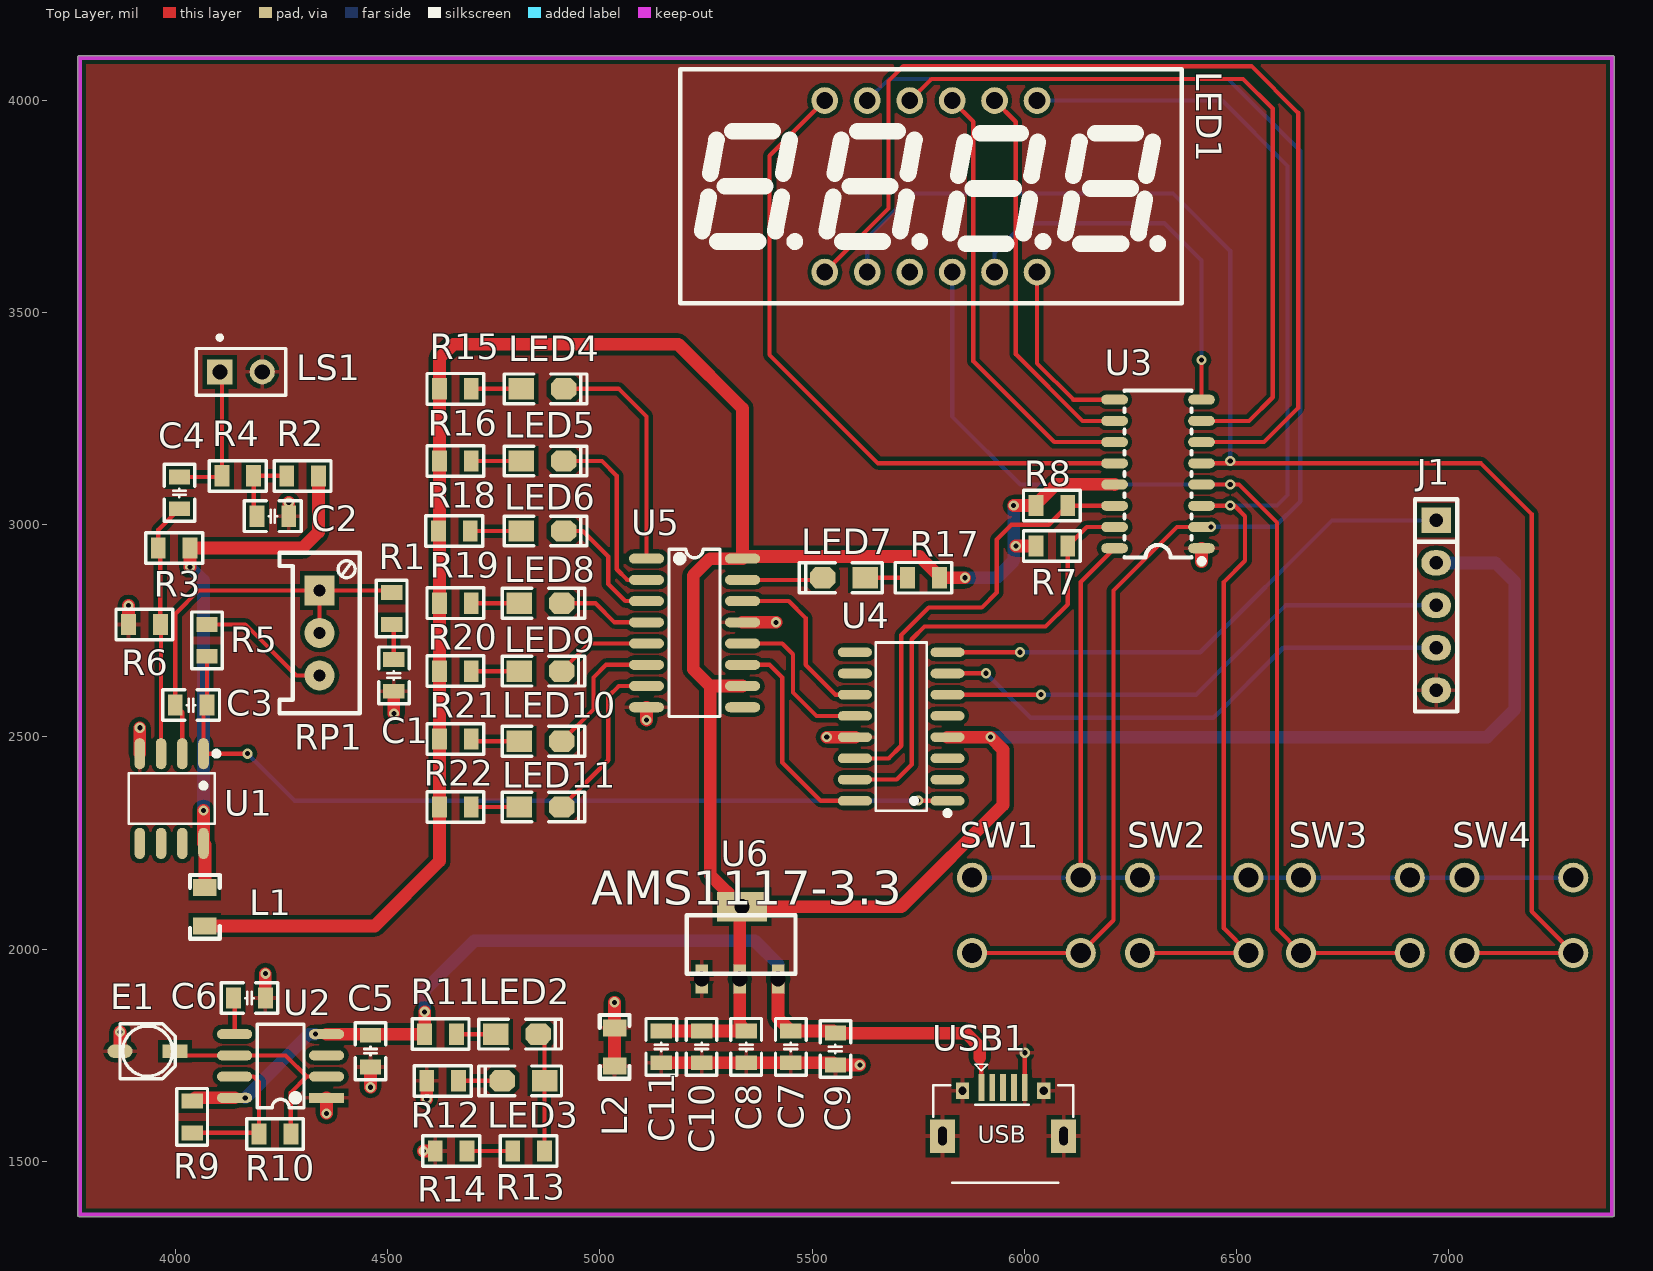
[diagram p0: Top Layer view]
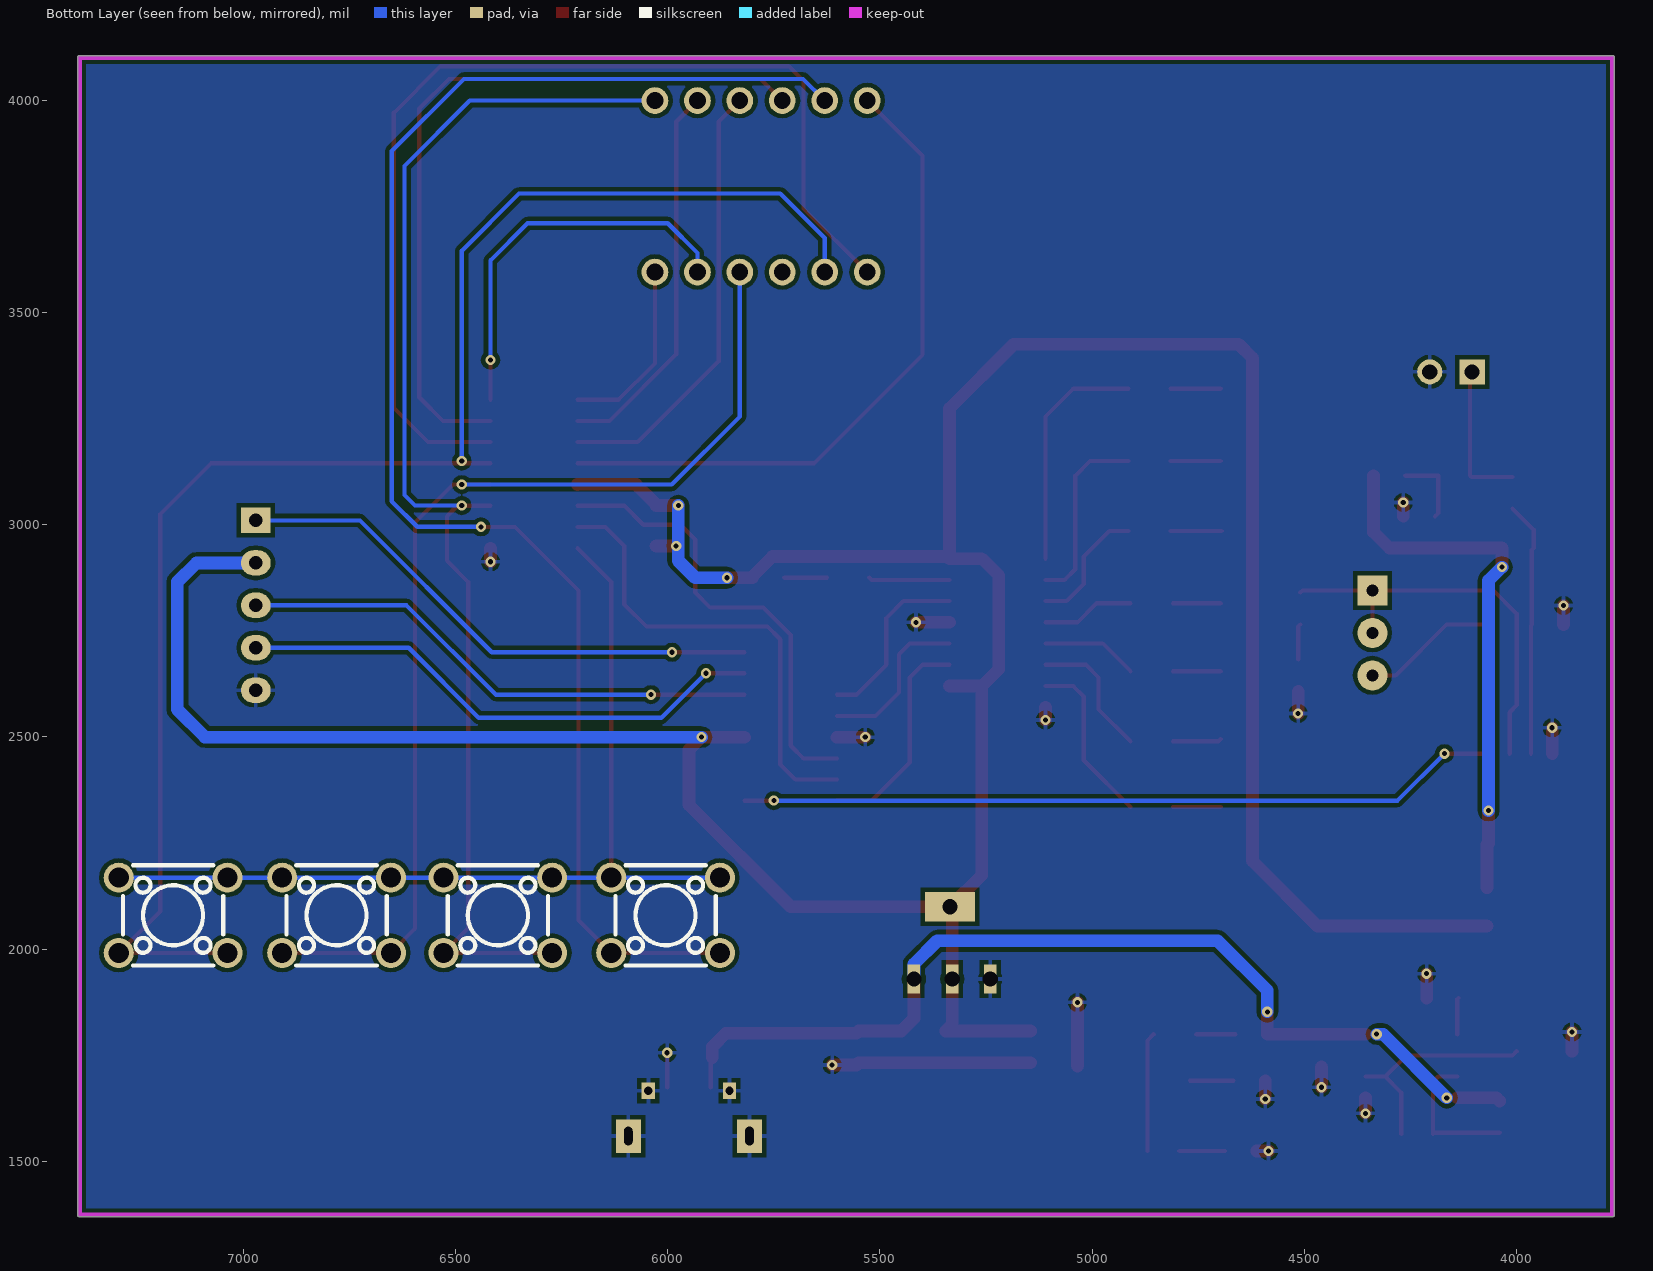
[diagram p1: Bottom Layer view, seen from below]
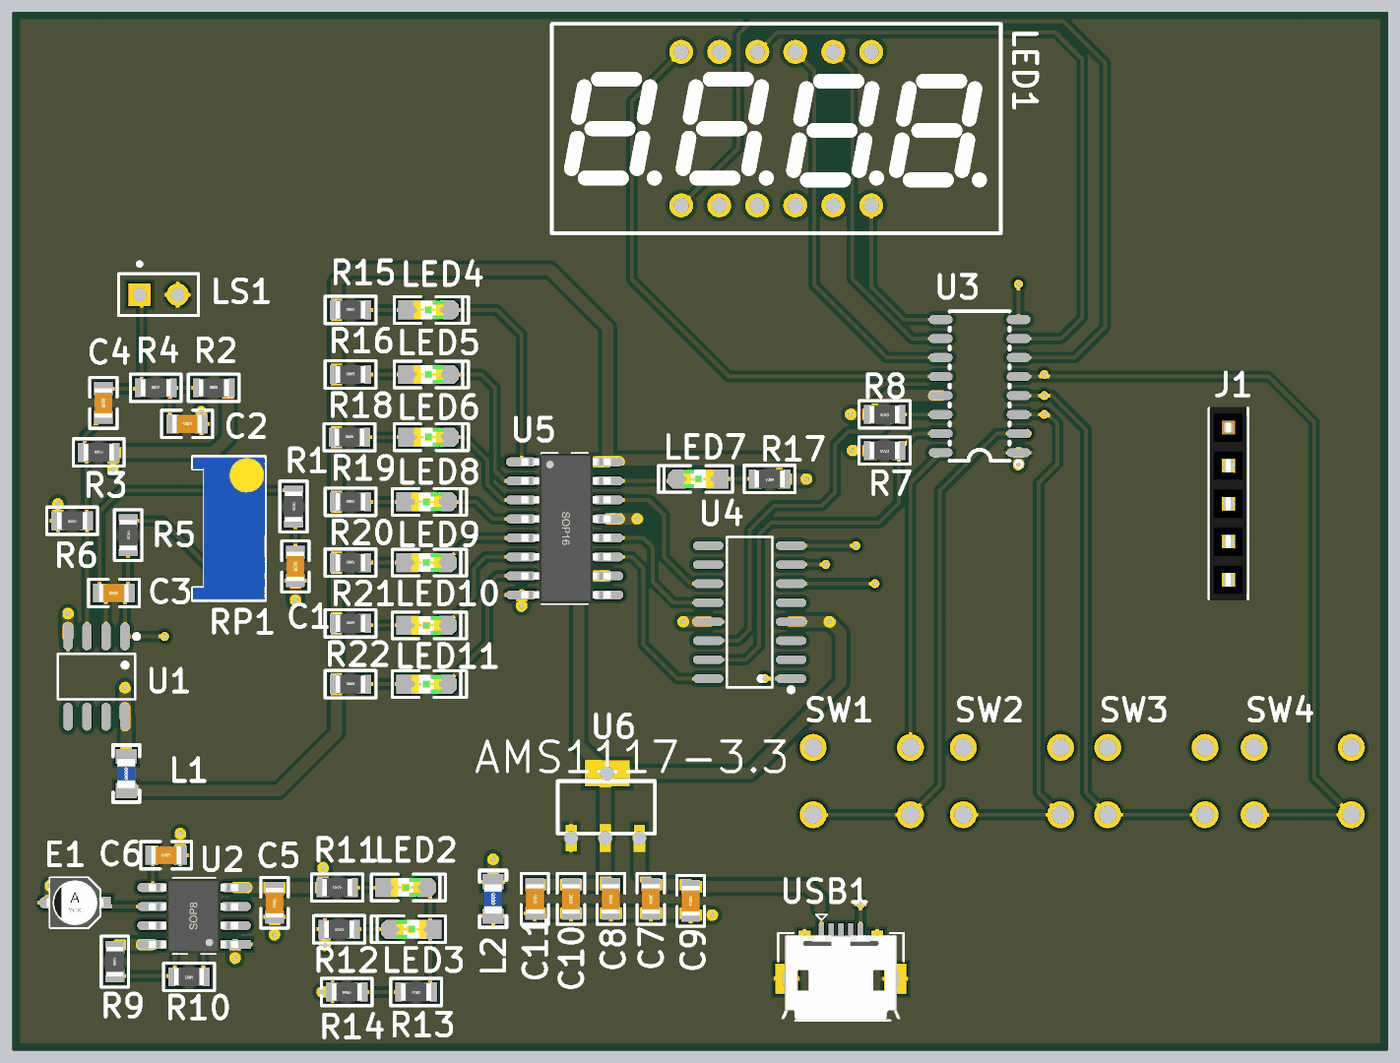
[diagram p2: 3D render of the assembled board from above, using the file's embedded part models]
# Altium PCB MISC80753.PcbDoc
Units mil, origin at the board's own origin, x right, y up, seen from the top; angles counter-clockwise.
Board outline 3620.03 x 2735.03 mil, 2 copper layers (Top Layer, Bottom Layer); 61 components, 56 nets, 207 pads, 36 vias.

## Layer stack, top to bottom (the 12.6 mil dielectric is the usual default, probably not edited)
Top Solder: solder mask 0.4, Solder Resist, Dk 3.5
Top Layer: signal copper 1.4
Dielectric 1: dielectric 12.6, FR-4, Dk 4.8
Bottom Layer: signal copper 1.4
Bottom Solder: solder mask 0.4, Solder Resist, Dk 3.5

## Board outline
3769.99,1375 ccw(c3775,1375) 3775,1369.98 7385,1369.98 ccw(c7385,1375) 7390.02,1375 7390.02,4100 ccw(c7385,4100) 7385,4105.02 3775,4105.02 ccw(c3775,4100) 3769.99,4100

## Design rules (kind name [scope] priority, off if disabled: settings)
Clearance [All] p1: gap=10
MinimumSolderMaskSliver [All] p1: minsoldermaskwidth=0
PolygonConnect [All] p1: connectstyle=Relief reliefconductorwidth=10 reliefentries=4 polygonreliefangle="90 Angle" airgapwidth=10
RoutingVias [All] p1: holewidth=28 width=50 viastyle="Through Hole" minholewidth=28 minwidth=50 maxholewidth=28 maxwidth=50
SilkToSilkClearance [All] p1: silktosilkclearance=0
SilkToSolderMaskClearance [IsPad] p1: minsilkscreentomaskgap=0 clearancetoexposedcopper=TRUE
SolderMaskExpansion [All] p1: expansion=4
Width [All] p1: maxlimit=30 minlimit=10 preferedwidth=10
27 further rules are at their usual default settings.

## Components (designator, comment, footprint, x,y, rotation, side; value= is the part's Value field where it differs from the comment)
C1 "10UF" "C 0805_L" 4515,2645 r270 top
C2 "0.1UF" "C 0805_L" 4230,3020 r180 top
C3 "100PF" "C 0805_L" 4037.4,2575 r0 top
C4 "0.01UF" "C 0805_L" 4010,3075 r270 top
C5 "10UF" "C 0805_L" 4460,1760 r90 top
C6 "10NF" "C 0805_L" 4175,1885 r0 top
C7 "100NF" "C 0805_L" 5450,1770 r90 top
C8 "100NF" "C 0805_L" 5345,1770 r90 top
C9 "10UF" "C 0805_L" 5555,1765 r90 top
C10 "10UF" "C 0805_L" 5240,1770 r90 top
C11 "100NF" "C 0805_L" 5145,1770 r90 top
E1 "10uF" "CM A(3*5.4)" 3935,1760 r0 top
J1 "Female HDR1X5" Fe-HDR1X5/2.54-S 6970,3010 r0 top
L1 "10uH" "L 0805" 4070,2100 r270 top
L2 "10uH" "L 0805" 5035,1770 r90 top
LED1 "SR410361N" LED-SEG-TH_12P-L30.0-W14.0-P2.54-S10.26-BL 5780,3796.97 r0 top
LED2 "Red" "LED 0805G" 4805,1800 r0 top
LED3 "Red" "LED 0805G" 4820,1690 r180 top
LED4 "Red" "LED 0805G" 4865,3320 r0 top
LED5 "Red" "LED 0805G" 4865,3150 r0 top
LED6 "Red" "LED 0805G" 4865,2985 r0 top
LED7 "Red" "LED 0805G" 5575,2875 r180 top
LED8 "Red" "LED 0805G" 4860,2815 r0 top
LED9 "Red" "LED 0805G" 4860,2655 r0 top
LED10 "Red" "LED 0805G" 4860,2490 r0 top
LED11 "Red" "LED 0805G" 4860,2335 r0 top
LS1 "Bell" PIN2 4105,3360 r0 top
R1 "1K" "R 0805_L" 4510,2802.6 r270 top
R2 "1K" "R 0805_L" 4300,3115 r0 top
R3 "1M" "R 0805_L" 3997.6,2945 r0 top
R4 "1K" "R 0805_L" 4147.4,3115 r0 top
R5 "10K" "R 0805_L" 4075,2727.4 r270 top
R6 "1M" "R 0805_L" 3927.6,2765 r180 top
R7 "10K" "R 0805_L" 6065,2950 r180 top
R8 "10K" "R 0805_L" 6065,3045 r180 top
R9 "100K" "R 0805_L" 4040,1605 r90 top
R10 "200K" "R 0805_L" 4235,1565 r180 top
R11 "1K" "R 0805_L" 4625,1800 r0 top
R12 "1K" "R 0805_L" 4630,1690 r180 top
R13 "10K" "R 0805_L" 4832.4,1525 r180 top
R14 "25K" "R 0805_L" 4650,1525 r180 top
R15 "1K" "R 0805_L" 4660,3320 r0 top
R16 "1K" "R 0805_L" 4660,3150 r0 top
R17 "1K" "R 0805_L" 5762.6,2875 r180 top
R18 "1K" "R 0805_L" 4657.4,2985 r0 top
R19 "1K" "R 0805_L" 4660,2815 r0 top
R20 "1K" "R 0805_L" 4660,2655 r0 top
R21 "1K" "R 0805_L" 4660,2495 r0 top
R22 "1K" "R 0805_L" 4660,2335 r0 top
RP1 "10K" 3296W 4340,2745 r270 top
SW1 "6x6x5" 四脚轻触开关 6005,2080 r0 top
SW2 "6x6x5" 四脚轻触开关 6400,2080 r0 top
SW3 "6x6x5" 四脚轻触开关 6780,2080 r0 top
SW4 "6x6x5" 四脚轻触开关 7165,2080 r0 top
U1 "COS2333SRC" SOP-8_L4.9-W3.9-P1.27-LS6.0-BL 3995,2355 r180 top
U2 "NE555" SOP8 4356.54,1650 r180 top
U3 "GN1651" SOP-16_L9.9-W3.9-P1.27-LS6.1-BL 6315,3115 r90 top
U4 "PY32F002AW15S6TU" SOP-16_L9.9-W3.9-P1.27-LS6.0-BL 5710,2520 r90 top
U5 "74HC595D" SOP16 5110,2920 r0 top
U6 "AMS1117-3.3" AMS1117-3.3 5222.95,2040.28 r0 top
USB1 "USB-5P" USB-MICRO_A 5950,1560 r0 top

## Footprints (in the part's own frame and the unit in brackets; to place one, negate y for a bottom-side part, rotate by r counter-clockwise, add the part's x,y. Pads: shape width x height; smd on the part's side, far side on the other; paste and mask are expansions set on the pad)
3296W [mm] "Precise Multi-Winding Adjustable Resistor"
  rect 1.8x1.8 hole 0.7: 1(-2.54,0)
  round 1.8 hole 0.7: 2(0,0) 3(2.54,0)
  silkscreen extent -4.8,-2.4 4.8,2.4, body extent -4.75,-2.4 4.75,2.4, height 11.52
AMS1117-3.3 [mm]
  rect 0.74x1.75 hole 0.914 paste+0 mask+0.051: 1(0.444,-2.801) 2(2.719,-2.801) 3(5.005,-2.801)
  rect 3x1.75 hole 0.914 paste+0 mask+0.051: 4(2.846,1.517)
  silkscreen extent -0.46,-2.49 6.04,1.01
"C 0805_L" [mil] "无极性贴片电容"
  rect 35x50 smd: 1(-37.4,0) 2(37.4,0)
  silkscreen extent -67,-36 67,36, body extent -39,-24 39,24, height 20
"CM A(3*5.4)" [mm] "贴片电解电容，直径3mm，高5.4mm"
  rect 1.5x0.8 smd: 1(1.651,0)
  oval 1.5x0.8 smd: 2(-1.65,0)
  silkscreen extent -1.65,-1.65 1.65,1.65, body extent -1.9,-1.65 1.9,1.65, height 5.4
Fe-HDR1X5/2.54-S [mil]
  rect 70x60 hole 32: 1(0,0)
  oval 70x60 hole 32: 2(0,-100) 3(0,-200) 4(0,-300) 5(0,-400)
  silkscreen extent -50,-450 50,50, body extent -50,-455 48,55, height 126
"L 0805" [mil] "小功率贴片电感"
  rect 40x55 smd: 1(-45,0) 2(45,0)
  silkscreen extent -75,-35 75,35, body extent -39,-24 39,24, height 35
"LED 0805G" [mil] "绿色0805LED"
  rect 60x50 smd: 1(-50,0)
  oct 60x50 smd: 2(50,0)
  silkscreen extent -90,-35 105,35, body extent -39,-25 39,25, height 32
LED-SEG-TH_12P-L30.0-W14.0-P2.54-S10.26-BL [mm]
  round 1.6 hole 1 paste+0 mask+0.051: 1(-6.35,-5.13) 2(-3.81,-5.13) 3(-1.27,-5.13) 4(1.27,-5.13) 5(3.81,-5.13) 6(6.35,-5.13) 7(6.35,5.13) 8(3.81,5.13) 9(1.27,5.13) 10(-1.27,5.13) 11(-3.81,5.13) 12(-6.35,5.13)
  silkscreen extent -15,-7 15,7
PIN2 [mm] "Photosensitive Diode; 2 Leads"
  rect 1.5x1.5 hole 0.9: 1(0,0)
  round 1.5 hole 0.9: 2(2.54,0)
  silkscreen extent -1.4,-1.4 3.94,2.17
"R 0805_L" [mil] "1/8W贴片电阻"
  rect 35x50 smd: 1(-37.4,0) 2(37.4,0)
  silkscreen extent -67,-36 67,36, body extent -39,-25 39,25, height 20
SOP8 [mm]
  rect 2.1x0.6 smd: 1(0,0)
  oval 2.1x0.6 smd: 2(0,-1.27) 3(0,-2.54) 4(0,-3.81) 5(5.5,-3.81) 6(5.5,-2.54) 7(5.5,-1.27) 8(5.5,0)
  silkscreen extent 1.35,-4.41 4.15,0.6, body extent -0.21,-4.4 5.8,0.6, height 1.9
SOP16 [mm]
  oval 2.1x0.6 smd: 1(0,0) 2(0,-1.27) 3(0,-2.54) 4(0,-3.81) 5(0,-5.08) 6(0,-6.35) 7(0,-7.62) 8(0,-8.89) 9(5.75,-8.89) 10(5.75,-7.62) 11(5.75,-6.35) 12(5.75,-5.08) 13(5.75,-3.81) 14(5.75,-2.54) 15(5.75,-1.27) 16(5.75,0)
  silkscreen extent 1.35,-9.45 4.4,0.56, body extent -0.04,-9.45 5.97,0.56, height 1.9
SOP-8_L4.9-W3.9-P1.27-LS6.0-BL [mm]
  oval 0.63x1.865 smd paste+0 mask+0.051: 1(-1.82,-2.682) 2(-0.55,-2.682) 3(0.72,-2.682) 4(1.99,-2.682) 5(1.99,2.682) 6(0.72,2.682) 7(-0.55,2.682) 8(-1.82,2.682)
  silkscreen extent -2.74,-2.83 2.66,1.52
SOP-16_L9.9-W3.9-P1.27-LS6.0-BL [mil]
  oval 22.6x80.24 smd paste+0 mask+2: 1(-170.43,-109.02) 2(-120.43,-109.02) 3(-70.43,-109.02) 4(-20.43,-109.02) 5(29.57,-109.02) 6(79.57,-109.02) 7(129.57,-109.02) 8(179.57,-109.02) 9(179.57,109.02) 10(129.57,109.02) 11(79.57,109.02) 12(29.57,109.02) 13(-20.43,109.02) 14(-70.43,109.02) 15(-120.43,109.02) 16(-170.43,109.02)
  silkscreen extent -205,-115 202,60
SOP-16_L9.9-W3.9-P1.27-LS6.1-BL [mm]
  oval 0.6x1.6 smd paste+0 mask+0.051: 1(-4.331,-2.6) 2(-3.061,-2.6) 3(-1.791,-2.6) 4(-0.521,-2.6) 5(0.749,-2.6) 6(2.019,-2.6) 7(3.289,-2.6) 8(4.559,-2.6) 9(4.559,2.6) 10(3.289,2.6) 11(2.019,2.6) 12(0.749,2.6) 13(-0.521,2.6) 14(-1.791,2.6) 15(-3.061,2.6) 16(-4.331,2.6)
  silkscreen extent -5.24,-2.76 5.11,2
USB-MICRO_A [mm] "micro型USB ，5.7*7.8*2.5mm"
  rect 0.35x1.6 smd: 1(-1.3,2.9) 2(-0.65,2.9) 3(0,2.9) 4(0.65,2.9) 5(1.3,2.9)
  rect 1.5x2 hole 0.5 slot 1.1 at 90 deg: 5(-3.625,0) 5(3.625,0)
  rect 0.8x1 hole 0.5: 5(-2.425,2.71) 5(2.425,2.71)
  silkscreen extent -4.19,-2.79 4.19,4.3, body extent -4,-2.71 4,2.89, height 2.8
四脚轻触开关 [mm]
  round 1.8 hole 1.2 paste+0 mask+0.102: 1(3.25,2.25) 2(-3.25,2.25) 3(3.25,-2.25) 4(-3.25,-2.25)

## Part data
C1 C2 C3 C4 C5 C6 C7 C8 C9 C10 C11: library part C, "Chip capacitor"
E1: library part CE_SMD, "Chip electrolytic capacitor"
L1 L2: library part L, "Low-power chip inductor"
LED2 LED3 LED4 LED5 LED6 LED7 LED8 LED9 LED10 LED11: library part LED-SMD, "Chip LED"
LS1: "Electrical Bell"
R1 R2 R3 R4 R5 R6 R7 R8 R9 R10 R11 R12 R13 R14 R15 R16 R17 R18 R19 R20 R21 R22: library part R, "Chip resistor"
RP1: library part RP, "Single-gang potentiometer"
SW1 SW2 SW3 SW4: library part "TSW DIP-6x6", "Through-hole 6x6 tactile switch"
U2: library part NE555D, "General-Purpose Single Bipolar Timer"
U5: library part SN74HC595D, "8-Bit Shift Register with 3-State Output Registers"
USB1: "Micro USB female socket"

## Via types
v1: diameter 24, hole 12, Top Layer to Bottom Layer, 36 vias

## Nets (pads, with @x,y where several pads share a name; then routed paths per layer and width w, separated by ;. In a path a pad name is that pad's centre, name@x,y a point inside that pad or via, vN(x,y) a via of type N, cw(c..) or ccw(c..) an arc to the next point about the centre after c; other vN are vias at no path point)
3V3: C8.2 C10.2 C11.2 J1.2 L1.2 R7.2 R8.2 R15.1 R16.1 R17.1 R18.1 R19.1 R20.1 R21.1 R22.1 U3.13 U4.4 U5.10 U5.16 U6.2 U6.4 | length 8351.1
  Top Layer w30: L1.2 4470,2055 4622.6,2207.6 R22.1 R21.1 R20.1 R19.1 R16.1 R15.1 4622.6,3392.6 4655,3425 5185,3425 5336.38,3273.62 U5.16@5336.38,2925 ; C11.2 C10.2 C8.2 5330,1822.4 U6.2 5330,2095 U6.4 ; U5.10 5260,2620 ; U4.4 v1(5920.43,2499.57) 5950,2470 5950,2340 5710,2100 U6.4 ; v1(5860,2875) R17.1 5800,2878.05 5753.05,2925 U5.16@5336.38,2925 ; v1(5975,3045) R8.2 6027.6,3048.06 6074.55,3095 6212.64,3095 U3.13 ; v1(5980,2950) R7.2 ; 5260,2620 5260,2175 U6.4 ; 5260,2620 5220,2660 5220,2880 5260,2920 U5.16 U5.16@5336.38,2925
  Bottom Layer w30: v1(5860,2875) 5935,2875 5975,2915 v1(5975,3045) ; v1(5920.43,2499.57) 7089.57,2499.57 7155,2565 7155,2865 7110,2910 J1.2
5V: C5.2 C7.2 C9.2 R9.2 R11.1 U2.4 U2.8 U6.3 USB1.1 | length 2295.7
  Top Layer w10: 5895,1745 5898.82,1741.18 USB1.1
  Top Layer w30: R9.2 4047.6,1650 U2.8 ; U2.4 R11.1 v1(4587.6,1852.6) ; U6.3 5420,1837.4 C7.2 5550,1807.4 C9.2 5862.6,1802.4 5895,1770 5895,1745
  Bottom Layer w30: v1(4165,1650) 4315,1800 v1(4330,1800) ; v1(4587.6,1852.6) 4587.6,1902.6 4705,2020 5365,2020 5420,1965 U6.3
ADC_IN: C3.2 R5.2 U1.1 U4.1 | length 2031.2
  Top Layer w10: R5.2 4074.8,2689.8 C3.2 4066.65,2566.85 U1.1 v1(4170.61,2460.61) ; v1(5750,2350) 5750.43,2349.57 U4.1
  Bottom Layer w10: v1(4170.61,2460.61) 4281.22,2350 v1(5750,2350)
AVCC: L1.1 R2.2 R3.2 U1.8 | length 1265
  Top Layer w30: v1(4035,2900) R3.2 4300,2945 4337.4,2982.4 R2.2 ; v1(4066.65,2326.65) U1.8 4070,2246.04 L1.1
  Bottom Layer w30: v1(4035,2900) 4066.65,2868.35 v1(4066.65,2326.65)
CLK: R7.1 U3.15 U4.15 | length 1111.5
  Top Layer w10: U4.15 5699.57,2399.57 5735,2435 5735,2730 5765,2760 6050,2760 6102.4,2812.4 R7.1 6146.9,2994.5 U3.15
DG1: LED1.12 U3.12 | length 1571.3
  Top Layer w10: LED1.12 5400,3868.95 5400,3400 5655.5,3144.5 U3.12
DG2: LED1.9 U3.11 | length 1046.2
  Top Layer w10: LED1.9 5880,3948.95 5880,3385 6070.5,3194.5 U3.11
DG3: LED1.8 U3.10 | length 915.7
  Top Layer w10: LED1.8 5980,3948.95 5980,3401.72 6137.21,3244.5 U3.10
DG4: LED1.6 U3.9 | length 433
  Top Layer w10: LED1.6 6030,3380 6115.5,3294.5 U3.9
DIO: R8.1 U3.14 U4.14 | length 1084.5
  Top Layer w10: U4.14 5680.43,2449.57 5710,2479.14 5710,2740 5775,2805 5900,2805 5935,2840 5935,2965 5970,3000 6057.4,3000 R8.1 6102.9,3044.5 U3.14
GND: C1.2 C2.1 C5.1 C6.2 C7.1 C8.1 C9.1 C10.1 C11.1 E1.2 J1.5 L2.1 L2.2 LS1.2 R6.2 R12.2 R14.2 U1.4 U2.1 U3.1 U4.13 U5.8 U5.13 U6.1 USB1.5 | length 1356.2
  Top Layer w10: USB1.5@6001.18,1674.17 v1(6001.18,1756.18)
  Top Layer w30: E1.2 v1(3870.04,1805.04) ; R6.2 v1(3890.2,2809.8) ; U1.4 v1(3916.65,2521.65) ; C6.2 v1(4212.4,1942.4) ; C2.1 v1(4267.4,3052.4) ; v1(4356.54,1613.46) U2.1 ; v1(4460,1675) C5.1 ; v1(4515,2555) C1.2 ; v1(4585,1525) R14.2 ; v1(4592.6,1647.4) R12.2 ; L2.1 L2.2 v1(5035,1875) ; v1(5110,2540) U5.8 ; C11.1 C10.1 C8.1 C7.1 5550,1732.6 C9.1 v1(5612.6,1727.6) ; U5.13 v1(5415,2770) ; v1(5534.57,2499.57) U4.13 ; v1(6417.36,2912.64) U3.1
K1: SW1.1 SW1.2 SW2.1 SW2.2 SW3.1 SW3.2 SW4.1 SW4.2 U3.16 | length 2224.8
  Top Layer w10: SW1.1 6132.95,2864.82 U3.16
  Bottom Layer w10: SW1.2 SW1.1 SW2.2 SW2.1 SW3.2 SW3.1 SW4.2 SW4.1
NetC1_1: C1.1 R1.2 | length 84.9
  Top Layer w10: R1.2 4515,2760.2 C1.1
NetC2_2: C2.2 R2.1 R4.2 | length 176
  Top Layer w10: C2.2 4184.8,3027.8 R4.2 R2.1
NetC3_1: C3.1 R1.1 RP1.1 RP1.2 U1.2 | length 971.1
  Top Layer w10: U1.2 4016.65,2558.35 C3.1 4000,2790 4055,2845 RP1.1 ; RP1.2 RP1.1 ; R1.1 4505,2845 RP1.1
NetC4_1: C4.1 LS1.1 R4.1 | length 348.1
  Top Layer w10: C4.1 4107.4,3112.4 R4.1 4110,3355 LS1.1
NetC4_2: C4.2 R3.1 R6.1 U1.3 | length 600.3
  Top Layer w10: U1.3 3966.65,2763.35 R6.1 3965,2940.2 R3.1 3960.2,2987.8 C4.2
NetC6_1: C6.1 U2.5 | length 86
  Top Layer w10: C6.1 4140,1882.59 U2.5
NetLED2_1: LED2.1 R11.2 | length 92.6
  Top Layer w10: R11.2 LED2.1
NetLED2_2: LED2.2 LED3.1 R13.1 | length 281.3
  Top Layer w10: LED2.2 4870,1785 LED3.1 4869.8,1689.8 R13.1
NetLED3_2: LED3.2 R12.1 | length 102.6
  Top Layer w10: R12.1 LED3.2
NetLED4_1: LED4.1 R15.2 | length 117.6
  Top Layer w10: R15.2 LED4.1
NetLED4_2: LED4.2 U5.1 | length 556.9
  Top Layer w10: LED4.2 5045,3320 5110,3255 U5.1
NetLED5_1: LED5.1 R16.2 | length 117.6
  Top Layer w10: R16.2 LED5.1
NetLED5_2: LED5.2 U5.2 | length 439.9
  Top Layer w10: LED5.2 5005,3150 5040,3115 5040,2895 5065,2870 U5.2
NetLED6_1: LED6.1 R18.2 | length 120.2
  Top Layer w10: R18.2 LED6.1
NetLED6_2: LED6.2 U5.3 | length 301.4
  Top Layer w10: LED6.2 4960,2985 5020,2925 5020,2860 5060,2820 U5.3
NetLED7_1: LED7.1 R17.2 | length 100.2
  Top Layer w10: LED7.1 R17.2
NetLED7_2: LED7.2 U5.15 | length 190.7
  Top Layer w10: U5.15 5520,2870 LED7.2
NetLED8_1: LED8.1 R19.2 | length 112.6
  Top Layer w10: R19.2 LED8.1
NetLED8_2: LED8.2 U5.4 | length 218.6
  Top Layer w10: LED8.2 4990,2815 5035,2770 U5.4
NetLED9_1: LED9.1 R20.2 | length 112.6
  Top Layer w10: R20.2 LED9.1
NetLED9_2: LED9.2 U5.5 | length 226.9
  Top Layer w10: LED9.2 4975,2720 U5.5
NetLED10_1: LED10.1 R21.2 | length 114.7
  Top Layer w10: R21.2 4702.4,2490 LED10.1
NetLED10_2: LED10.2 U5.6 | length 318.5
  Top Layer w10: LED10.2 4985,2565 4985,2640 5015,2670 U5.6
NetLED11_1: LED11.1 R22.2 | length 112.6
  Top Layer w10: R22.2 LED11.1
NetLED11_2: LED11.2 U5.7 | length 405.9
  Top Layer w10: LED11.2 5020,2445 5020,2595 5045,2620 U5.7
NetR5_1: R5.1 RP1.3 | length 314.6
  Top Layer w10: R5.1 4165.2,2764.8 4285,2645 RP1.3
NetR9_1: R9.1 R10.2 U2.7 | length 343.9
  Top Layer w10: R9.1 4195.01,1567.6 R10.2 4197.6,1687.4 4185,1700 U2.7
NetR13_2: R13.2 R14.1 | length 107.6
  Top Layer w10: R14.1 R13.2
NRST: J1.1 U4.8 | length 1279.6
  Top Layer w10: U4.8 v1(5989.57,2699.57)
  Bottom Layer w10: v1(5989.57,2699.57) 6414.57,2699.57 6725,3010 J1.1
O_555: U2.3
PA0: U4.11 U5.14 | length 420.3
  Top Layer w10: U5.14 5445,2820 5485,2780 5485,2670 5555.43,2599.57 U4.11
PA1: U4.12 U5.12 | length 387.9
  Top Layer w10: U5.12 5430,2720 5455,2695 5455,2605 5510.43,2549.57 U4.12
PA6: U4.16 U5.11 | length 514.5
  Top Layer w10: U5.11 5400,2670 5430,2640 5430,2440 5520.43,2349.57 U4.16
PB0: U4.2
RC: E1.1 R10.1 U2.2 U2.6 | length 532
  Top Layer w10: E1.1 4010,1750 U2.6 4260,1750 4310,1700 ; R10.1 4272.4,1662.4 4310,1700 ; U2.2 4310,1700
SG1: LED1.11 SW1.3 SW1.4 U3.2 | length 3605
  Top Layer w10: SW1.4 SW1.3 6210,2068.46 6210,2845 6359.5,2994.5 U3.2 6439.5,2994.5 v1(6440,2995)
  Bottom Layer w10: LED1.11 5681.05,4050 6480,4050 6650,3880 6650,3055 6590,2995 v1(6440,2995)
SG2: LED1.7 SW2.3 SW2.4 U3.3 | length 3016.1
  Top Layer w10: SW2.4 SW2.3 6470,2049.37 6470,2865 6520,2915 6520,3020 6495.5,3044.5 U3.3
  Bottom Layer w10: LED1.7 6466.05,3998.95 6620,3845 6620,3070 6595,3045 v1(6485,3045)
SG3: LED1.4 SW3.3 SW3.4 U3.4 | length 2569.3
  Top Layer w10: U3.4 v1(6485,3094.5) 6505.5,3094.5 6595,3005 6595,2048.46 SW3.4 SW3.3
  Bottom Layer w10: LED1.4 5830,3255 5990.5,3094.5 v1(6485,3094.5)
SG4: LED1.2 SW4.3 SW4.4 U3.5 | length 3686.6
  Top Layer w10: U3.5 7075.5,3144.5 7195,3025 7195,2089.37 SW4.3 SW4.4
  Bottom Layer w10: LED1.2 5630,3675 5735,3780 6350,3780 6485,3645 v1(6485,3150)
SG5: LED1.1 U3.6 | length 2493.2
  Top Layer w10: LED1.1 5680,3745 5680,4045 5715,4080 6535,4080 6645,3970 6645,3275 6564.5,3194.5 U3.6
SG6: LED1.10 U3.7 | length 1775.8
  Top Layer w10: LED1.10 5781.05,4050 6515,4050 6585,3980 6585,3300 6529.5,3244.5 U3.7
SG7: LED1.5 U3.8 | length 929
  Top Layer w10: v1@6415,3390 v1(6417.36,3387.64) U3.8
  Bottom Layer w10: LED1.5 5930,3640 6000,3710 6330,3710 6417.36,3622.64 v1(6417.36,3387.64)
SWC: J1.4 U4.7 | length 1263
  Top Layer w10: U4.7 5819.45,2650 v1(5910,2650)
  Bottom Layer w10: v1(5910,2650) 6015,2545 6445,2545 6610,2710 J1.4
SWD: J1.3 U4.6 | length 1238.1
  Top Layer w10: U4.6 v1(6039.57,2599.57)
  Bottom Layer w10: v1(6039.57,2599.57) 6404.57,2599.57 6615,2810 J1.3
pads on no net: LED1.3 U1.5 U1.6 U1.7 U4.3 U4.5 U4.9 U4.10 U5.9 USB1.2 USB1.3 USB1.4

## Polygon pours and split planes (outlines as drawn)
GND on Bottom Layer "D" (solid, remove dead copper, pour order 2): 3515,4245 7635,4245 7735,4345 7645,4255 7645,950 3765,950 3535,1180
GND on Top Layer "D" (solid, remove dead copper, pour order 4): 3635,4145 3695,4205 7495,4205 7495,1390 7530,1355 7335,1160 3620,1160

## Keep-outs
Keep-Out Layer:
  lines w10: 7250,1375 7385,1375 7385,2185 ; 7275,1375 3775,1375 3775,4100 3825,4100 5225,4100 7385,4100 7385,3975 ; 7385,2175 7385,4000